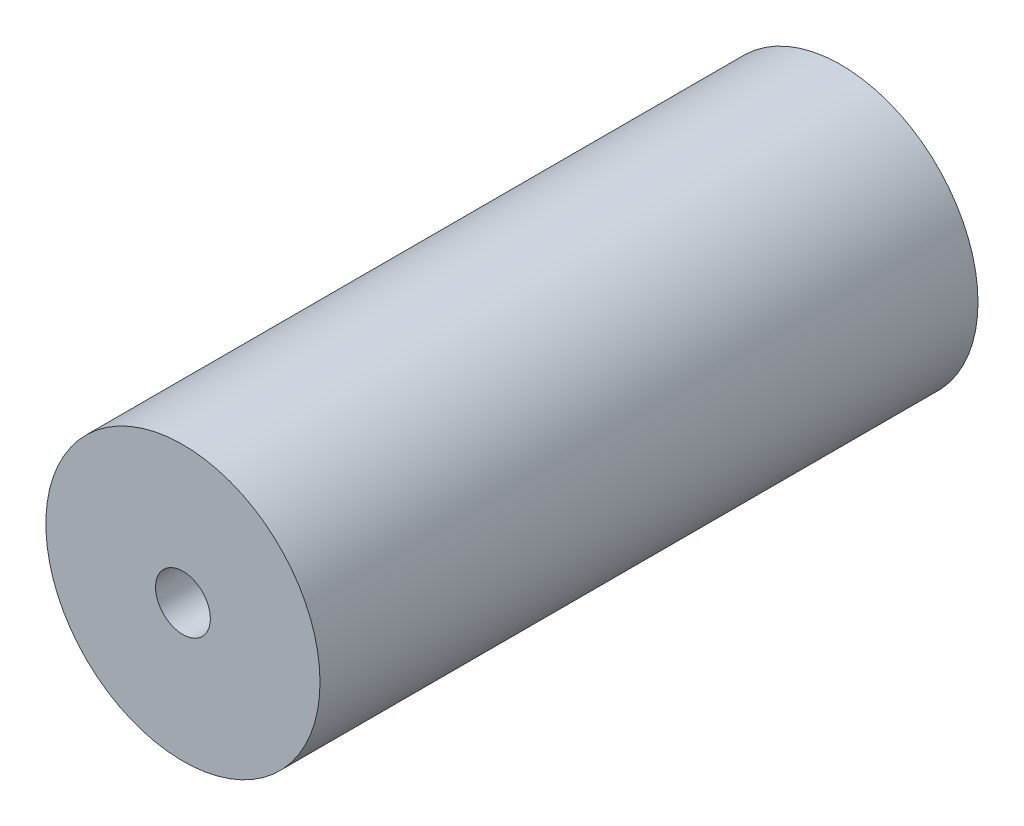
from build123d import *

# Parameters (mm, degrees)
SKETCH_1_R             = 12.5
BOSS_EXTRUDE_1_DEPTH   = 60
M6_TAPPED_HOLE_1_D     = 5
M6_TAPPED_HOLE_1_DEPTH = 15
M6_TAPPED_HOLE_1_TIP   = 1.502151548
M6_TAPPED_HOLE_2_D     = 5
M6_TAPPED_HOLE_2_DEPTH = 15
M6_TAPPED_HOLE_2_TIP   = 1.502151548


with BuildPart() as part:
    # Sketch 1 → Boss-Extrude 1 (new body)
    with BuildSketch(Plane.XY):
        Circle(SKETCH_1_R)
    extrude(amount=BOSS_EXTRUDE_1_DEPTH)

    # M6 Tapped Hole 1
    with Locations(Plane.XY.offset(60)):
        with Locations((0, 0)):
            Hole(M6_TAPPED_HOLE_1_D / 2, depth=M6_TAPPED_HOLE_1_DEPTH)
            with Locations((0, 0, -(M6_TAPPED_HOLE_1_DEPTH + M6_TAPPED_HOLE_1_TIP / 2))):  # 118° drill point
                Cone(0, M6_TAPPED_HOLE_1_D / 2, M6_TAPPED_HOLE_1_TIP, mode=Mode.SUBTRACT)

    # M6 Tapped Hole 2
    with Locations(Plane(origin=(0, 0, 0), x_dir=(-1, 0, 0), z_dir=(0, 0, -1))):
        with Locations((0, 0)):
            Hole(M6_TAPPED_HOLE_2_D / 2, depth=M6_TAPPED_HOLE_2_DEPTH)
            with Locations((0, 0, -(M6_TAPPED_HOLE_2_DEPTH + M6_TAPPED_HOLE_2_TIP / 2))):  # 118° drill point
                Cone(0, M6_TAPPED_HOLE_2_D / 2, M6_TAPPED_HOLE_2_TIP, mode=Mode.SUBTRACT)


solid = part.part
